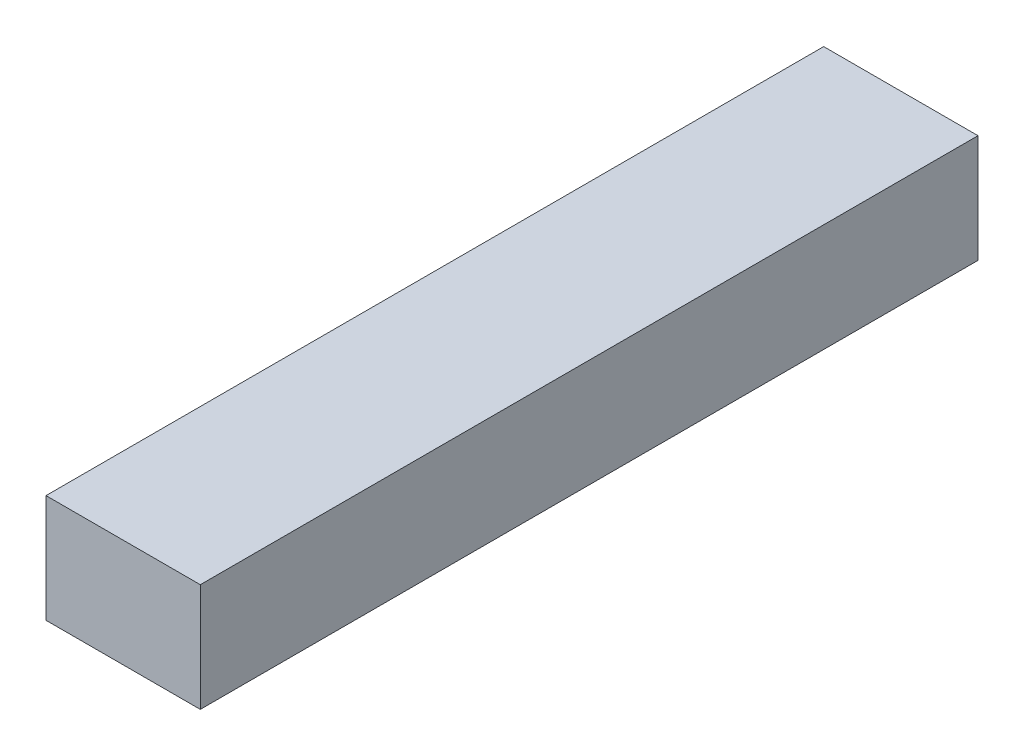
from build123d import *

# Parameters (mm, degrees)
SKETCH2_W           = 25
SKETCH2_H           = 126
BOSS_EXTRUDE1_DEPTH = 8.75


with BuildPart() as part:
    # Sketch2 → Boss-Extrude1 (new, symmetric)
    with BuildSketch(Plane(origin=(0, 0, 0), x_dir=(1, 0, 0), z_dir=(0, 1, 0))):
        Rectangle(SKETCH2_W, SKETCH2_H)
    extrude(amount=BOSS_EXTRUDE1_DEPTH, both=True)


solid = part.part
